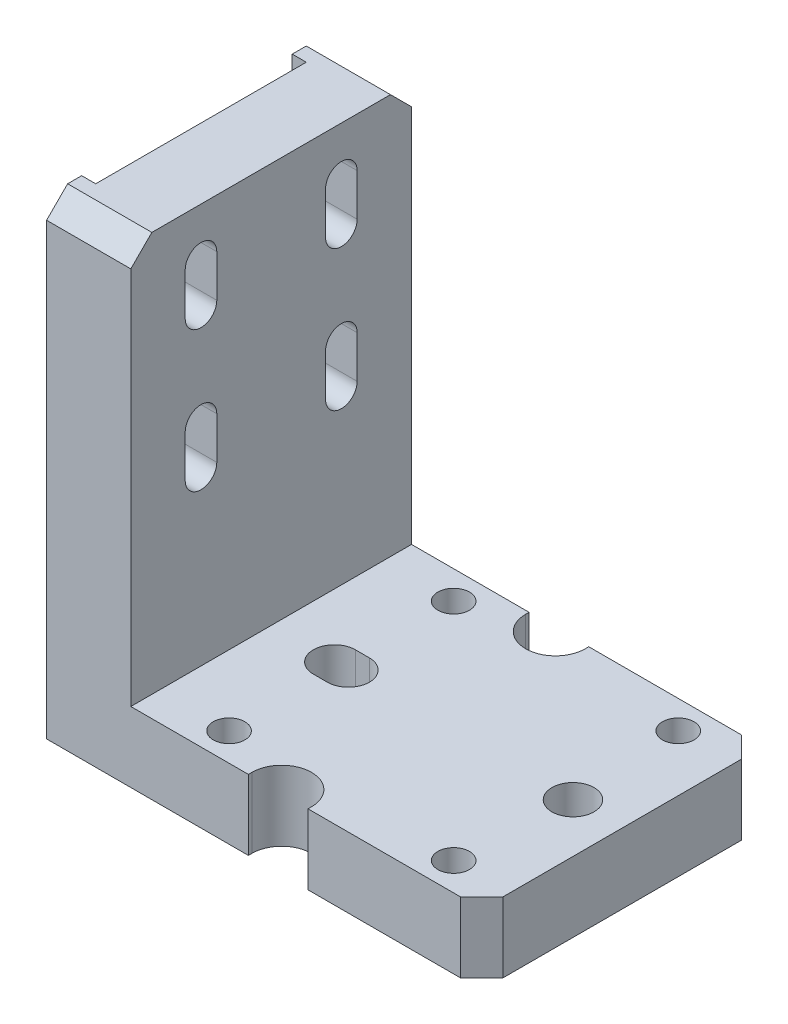
from build123d import *

# Parameters (mm, degrees)
SKETCH1_W                  = 62
SKETCH1_H                  = 67
BOSS_EXTRUDE1_DEPTH        = 20
SKETCH2_W                  = 50
SKETCH2_H                  = 57
CUT_EXTRUDE1_DEPTH         = 61.689784972
SKETCH3_W                  = 2
SKETCH3_H                  = 30
CUT_EXTRUDE2_DEPTH         = 77.485292704
CUT_EXTRUDE3_DEPTH         = 64.421210963
F_4_5_4_5_DIAMETER_HOLE1_D = 4.5
SKETCH7_R                  = 3
CUT_EXTRUDE4_DEPTH         = 68.896980787
CHAMFER1_SIZE              = 3
CUT_EXTRUDE5_DEPTH         = 68.896980787


with BuildPart() as part:
    # Sketch1 → Boss-Extrude1 (new, symmetric)
    with BuildSketch(Plane.XY):
        Rectangle(SKETCH1_W, SKETCH1_H)
    extrude(amount=BOSS_EXTRUDE1_DEPTH, both=True)

    # Sketch2 → Cut-Extrude1 (cut, through all)
    with BuildSketch(Plane.XY.offset(20)):
        with Locations((6, 5)):
            Rectangle(SKETCH2_W, SKETCH2_H)
    extrude(amount=-CUT_EXTRUDE1_DEPTH, mode=Mode.SUBTRACT)

    # Sketch3 → Cut-Extrude2 (cut, through all)
    with BuildSketch(Plane(origin=(0, 33.5, 0), x_dir=(1, 0, 0), z_dir=(0, 1, 0))):
        with Locations((-30, 0)):
            Rectangle(SKETCH3_W, SKETCH3_H)
    extrude(amount=-CUT_EXTRUDE2_DEPTH, mode=Mode.SUBTRACT)

    # Sketch4 → Cut-Extrude3 (cut, through all)
    with BuildSketch(Plane(origin=(-19, 0, 0), x_dir=(0, 0, -1), z_dir=(1, 0, 0))):
        with BuildLine():
            Line((-7.75, 26.5), (-7.75, 20.5))
            ThreePointArc((-7.75, 20.5), (-10, 18.25), (-12.25, 20.5))
            Line((-12.25, 20.5), (-12.25, 26.5))
            ThreePointArc((-12.25, 26.5), (-10, 28.75), (-7.75, 26.5))
        make_face()
        with BuildLine():
            Line((-7.75, 6.5), (-7.75, 0.5))
            ThreePointArc((-7.75, 0.5), (-10, -1.75), (-12.25, 0.5))
            Line((-12.25, 0.5), (-12.25, 6.5))
            ThreePointArc((-12.25, 6.5), (-10, 8.75), (-7.75, 6.5))
        make_face()
        with BuildLine():
            Line((12.25, 26.5), (12.25, 20.5))
            ThreePointArc((12.25, 20.5), (10, 18.25), (7.75, 20.5))
            Line((7.75, 20.5), (7.75, 26.5))
            ThreePointArc((7.75, 26.5), (10, 28.75), (12.25, 26.5))
        make_face()
        with BuildLine():
            Line((12.25, 6.5), (12.25, 0.5))
            ThreePointArc((12.25, 0.5), (10, -1.75), (7.75, 0.5))
            Line((7.75, 0.5), (7.75, 6.5))
            ThreePointArc((7.75, 6.5), (10, 8.75), (12.25, 6.5))
        make_face()
    extrude(amount=-CUT_EXTRUDE3_DEPTH, mode=Mode.SUBTRACT)

    # Ø4.5 (4.5) Diameter Hole1 (through all)
    with Locations(Plane(origin=(0, -23.5, 0), x_dir=(1, 0, 0), z_dir=(0, 1, 0))):
        with Locations((-9, 16), (-9, -16), (23, -16), (23, 16)):
            Hole(F_4_5_4_5_DIAMETER_HOLE1_D / 2)

    # Sketch7 → Cut-Extrude4 (cut, through all)
    with BuildSketch(Plane(origin=(0, -23.5, 0), x_dir=(1, 0, 0), z_dir=(0, 1, 0))):
        with Locations(Location((24, 0, 0), (0, 0, 270))):
            Circle(SKETCH7_R)
        with BuildLine():
            Line((-10, 3), (-8, 3))
            ThreePointArc((-8, 3), (-5, 0), (-8, -3))
            Line((-8, -3), (-10, -3))
            ThreePointArc((-10, -3), (-13, 0), (-10, 3))
        make_face()
    extrude(amount=-CUT_EXTRUDE4_DEPTH, mode=Mode.SUBTRACT)

    # Chamfer1
    chamfer1_edges = [part.edges().sort_by_distance(p)[0] for p in [
        (-25, 33.5, -20),
        (-25, 33.5, 20),
        (31, -28.5, 20),
        (31, -28.5, -20),
    ]]
    chamfer(chamfer1_edges, length=CHAMFER1_SIZE)

    # Sketch8 → Cut-Extrude5 (cut, through all)
    with BuildSketch(Plane(origin=(0, -23.5, 0), x_dir=(1, 0, 0), z_dir=(0, 1, 0))):
        with BuildLine():
            Line((6.25, -19.5), (6.25, -27.0274699))
            ThreePointArc((6.25, -27.0274699), (2, -31.2774699), (-2.25, -27.0274699))
            Line((-2.25, -27.0274699), (-2.25, -19.5))
            ThreePointArc((-2.25, -19.5), (2, -15.25), (6.25, -19.5))
        make_face()
        with BuildLine():
            Line((-2.25, 19.5), (-2.25, 27.0274699))
            ThreePointArc((-2.25, 27.0274699), (2, 31.2774699), (6.25, 27.0274699))
            Line((6.25, 27.0274699), (6.25, 19.5))
            ThreePointArc((6.25, 19.5), (2, 15.25), (-2.25, 19.5))
        make_face()
    extrude(amount=-CUT_EXTRUDE5_DEPTH, mode=Mode.SUBTRACT)


solid = part.part
